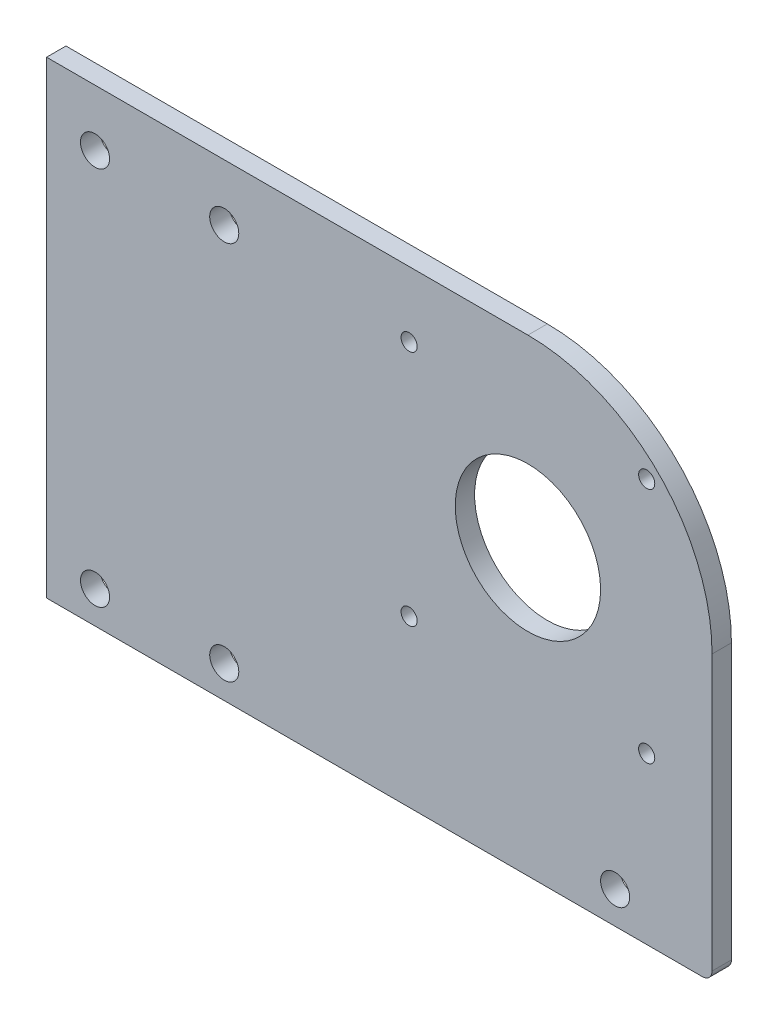
from build123d import *

# Parameters (mm, degrees)
SKETCH_1_W               = 206
SKETCH_1_H               = 145
EXTRUDE_1_DEPTH          = 6
SKETCH_3_R               = 4.5
CUT_EXTRUDE_2_DEPTH      = 127.100158604
SKETCH_4_R               = 22.5
CUT_EXTRUDE_3_DEPTH      = 127.100158604
FILLET_1_R               = 57
HOLE_WIZARD_M6_1_D       = 5
PATTERN_CIRCULAR_1_COUNT = 4
SKETCH_11_R              = 4.5
CUT_EXTRUDE_6_DEPTH      = 127.100158604
FILLET_5_R               = 3


with BuildPart() as part:
    # 草图1 → 凸台-拉伸1 (new body)
    with BuildSketch(Plane.XY):
        Rectangle(SKETCH_1_W, SKETCH_1_H)
    extrude(amount=EXTRUDE_1_DEPTH)

    # 草图3 → 切除-拉伸2 (cut, through all)
    with BuildSketch(Plane.XY.offset(6)):
        with Locations((-88, 55)):
            Circle(SKETCH_3_R)
        with Locations((-48, 55)):
            Circle(SKETCH_3_R)
        with Locations((-88, -62.5)):
            Circle(SKETCH_3_R)
        with Locations((-48, -62.5)):
            Circle(SKETCH_3_R)
    extrude(amount=-CUT_EXTRUDE_2_DEPTH, mode=Mode.SUBTRACT)

    # 草图4 → 切除-拉伸3 (cut, through all)
    with BuildSketch(Plane.XY.offset(6)):
        with Locations((46, 15.5)):
            Circle(SKETCH_4_R)
    extrude(amount=-CUT_EXTRUDE_3_DEPTH, mode=Mode.SUBTRACT)

    # 圆角1
    fillet_1_edges = [part.edges().sort_by_distance(p)[0] for p in [
        (103, 72.5, 3),
    ]]
    fillet(fillet_1_edges, radius=FILLET_1_R)

    # M6 螺纹孔1 (through all)
    with Locations(Plane.XY.offset(6)):
        with Locations((9.230447378, 52.269552622)):
            hole_wizard_m6_1 = Hole(HOLE_WIZARD_M6_1_D / 2)

    # 阵列(圆周)1: M6 螺纹孔1 ×4 about axis
    pattern_circular_1_axis = Axis((46, 15.5, 0), (0, 0, 1))
    for i in range(1, PATTERN_CIRCULAR_1_COUNT):
        add(hole_wizard_m6_1.rotate(pattern_circular_1_axis, i * 360 / PATTERN_CIRCULAR_1_COUNT), mode=Mode.SUBTRACT)

    # 草图11 → 切除-拉伸6 (cut, through all)
    with BuildSketch(Plane.XY.offset(6)):
        with Locations((73, -62.5)):
            Circle(SKETCH_11_R)
    extrude(amount=-CUT_EXTRUDE_6_DEPTH, mode=Mode.SUBTRACT)

    # 圆角5
    fillet_5_edges = [part.edges().sort_by_distance(p)[0] for p in [
        (103, -72.5, 3),
    ]]
    fillet(fillet_5_edges, radius=FILLET_5_R)


solid = part.part
